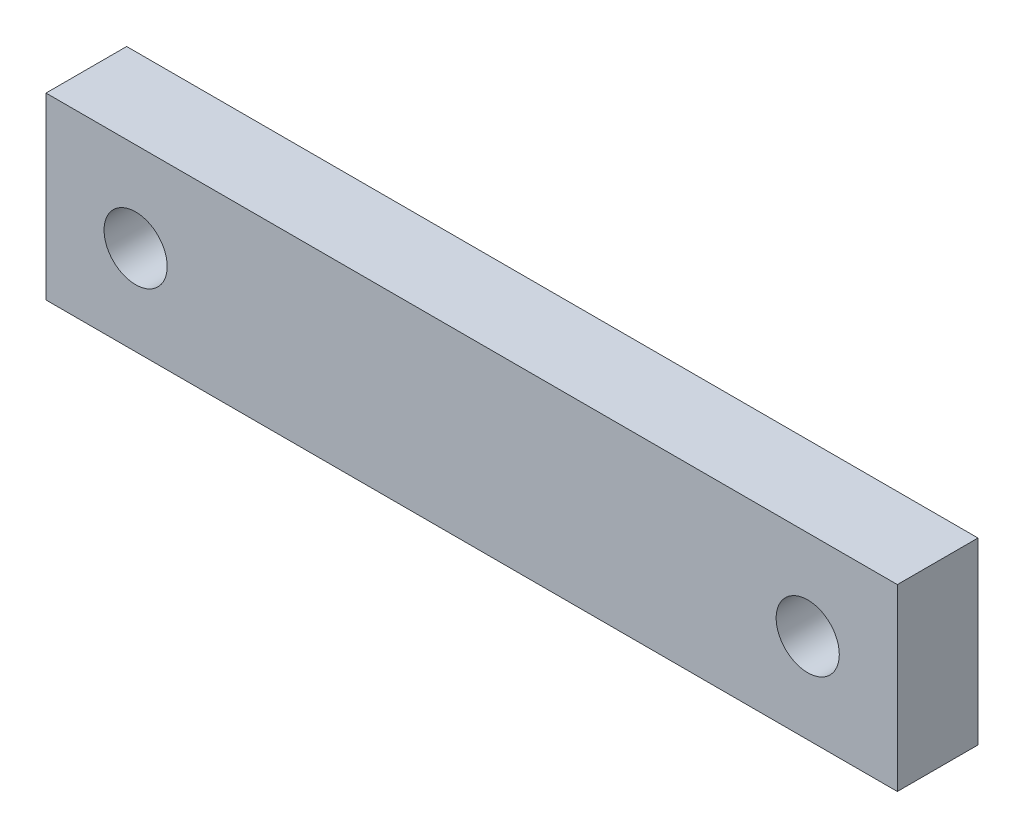
SolidWorks part; units mm, degrees
material "普通碳钢"
ref_plane "Front Plane" through (0, 0, 0) normal (0, 0, 1) x (1, 0, 0)
ref_plane "Top Plane" through (0, 0, 0) normal (0, 1, 0) x (1, 0, 0)
ref_plane "Right Plane" through (0, 0, 0) normal (1, 0, 0) x (0, 0, -1)
sketch "Sketch1" plane through (0, 0, 0) normal (0, 0, 1) x (1, 0, 0)
  line L1 (-190, 40) -> (190, 40)
  line L2 (-190, 40) -> (-190, -40)
  line L3 (-190, -40) -> (190, -40)
  line L4 (190, 40) -> (190, -40)
  dimension "D1" = 80
  dimension "D2" = 380
  dimension "D3" = 40
  dimension "D4" = 190
extrude "Boss-Extrude1" add sketch "Sketch1" along normal mid plane 36
hole_wizard "1-1/4-7 Tapped Hole1" positions "Sketch3" profile "Sketch2" tap size "1-1/4-7" standard "Ansi Inch" end condition through all
sketch "Sketch3" plane through (0, 0, 18) normal (0, 0, 1) x (1, 0, 0)
  line L0 (-190, 40) -> (-190, -40) construction
  line L1 (190, -40) -> (190, 40) construction
  point P0 (-150, 0)
  point P1 (150, 0)
  dimension "D1" = 40
  dimension "D2" = 40
sketch "Sketch2" plane through (-150, 0, 18) normal (1, 0, 0) x (0, -1, 0)
  line L0 (0, 0) -> (0, 36)
  line L1 (0, 36) -> (14.0894, 36)
  line L2 (14.0894, 36) -> (14.0894, 0)
  line L5 (14.0894, 0) -> (0, 0)
  line L11 (0, -6.35) -> (0, 107.95) construction
  dimension "通孔螺纹孔钻头直径" = 28.1788
  dimension "通孔螺纹孔钻头深度" = 36
cosmetic thread "Cosmetic thread1"
cosmetic thread "Cosmetic thread2"
